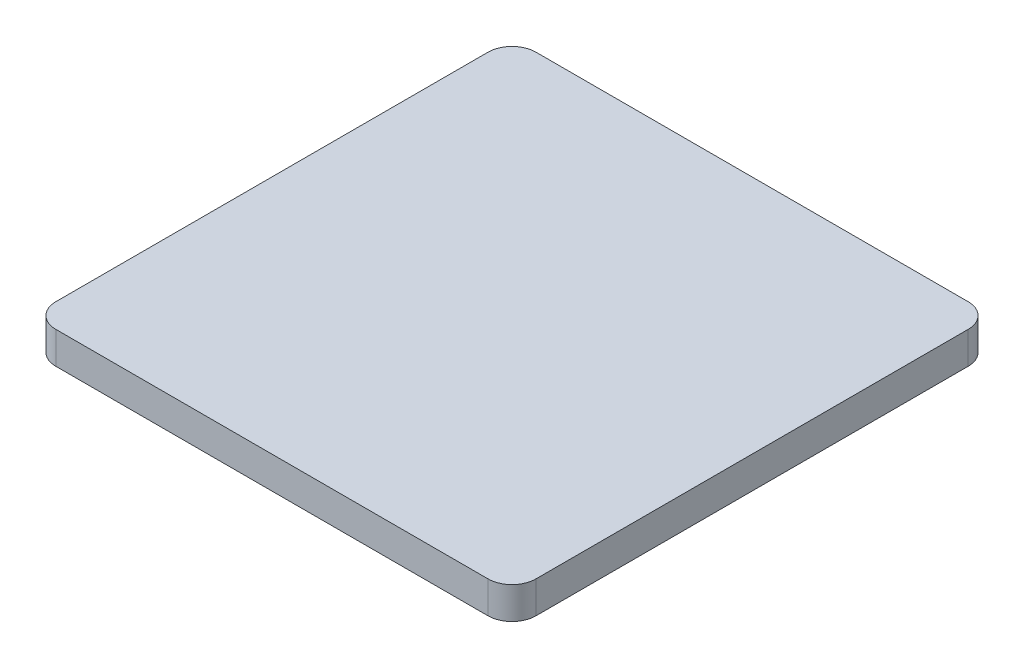
from build123d import *

# Parameters (mm, degrees)
BOSS_EXTRUDE_1_DEPTH = 20


with BuildPart() as part:
    # Sketch 1 → Boss-Extrude 1 (new body)
    with BuildSketch(Plane(origin=(0, 0, 0), x_dir=(1, 0, 0), z_dir=(0, 1, 0))):
        with BuildLine():
            Line((135, 150), (-135, 150))
            ThreePointArc((-135, 150), (-145.606601718, 145.606601718), (-150, 135))
            Line((-150, 135), (-150, -135))
            ThreePointArc((-150, -135), (-145.606601718, -145.606601718), (-135, -150))
            Line((-135, -150), (135, -150))
            ThreePointArc((135, -150), (145.606601718, -145.606601718), (150, -135))
            Line((150, -135), (150, 135))
            ThreePointArc((150, 135), (145.606601718, 145.606601718), (135, 150))
        make_face()
    extrude(amount=BOSS_EXTRUDE_1_DEPTH)


solid = part.part
